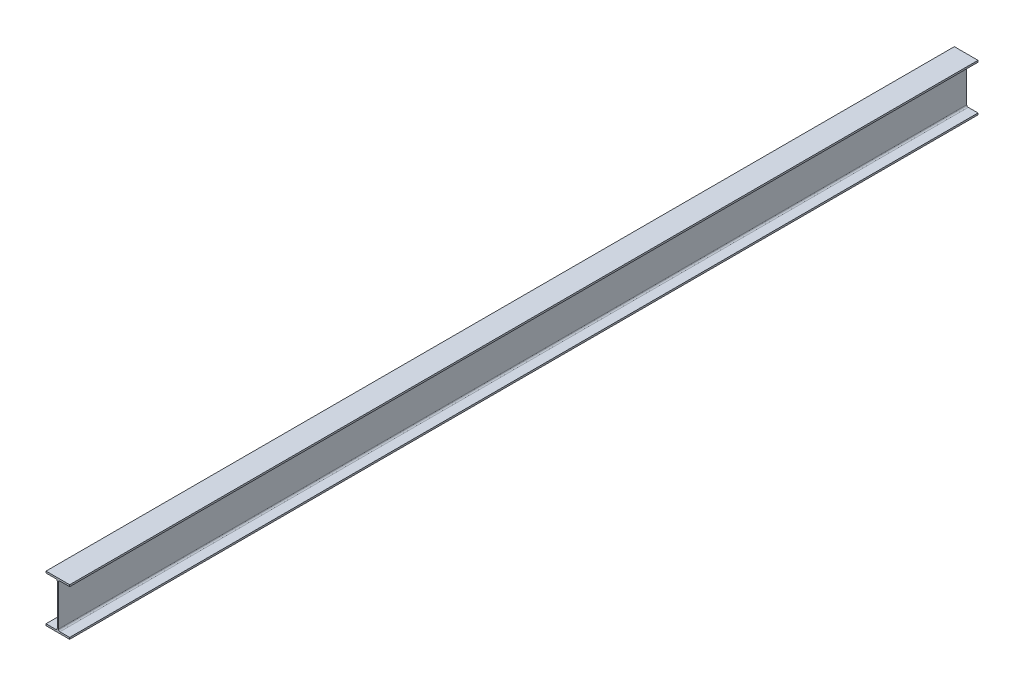
SolidWorks part; units mm, degrees
ref_plane "Front Plane" through (0, 0, 0) normal (0, 0, 1) x (1, 0, 0)
ref_plane "Top Plane" through (0, 0, 0) normal (0, 1, 0) x (1, 0, 0)
ref_plane "Right Plane" through (0, 0, 0) normal (1, 0, 0) x (0, 0, -1)
other "Configuration Table"
sketch "Sketch1" plane through (0, 0, 0) normal (0, 0, 1) x (1, 0, 0)
  line L0 (0, 0) -> (0, 250) construction
  line L1 (62.5, 0) -> (-62.5, 0)
  line L2 (-62.5, 0) -> (-62.5, 9)
  line L3 (-62.5, 9) -> (-11, 9)
  line L4 (3, 17) -> (3, 233)
  line L6 (-62.5, 241) -> (-62.5, 250)
  line L7 (-62.5, 250) -> (62.5, 250)
  line L8 (-3, 17) -> (-3, 233)
  line L9 (62.5, 241) -> (62.5, 250)
  line L10 (11, 241) -> (62.5, 241)
  line L11 (62.5, 9) -> (11, 9)
  line L12 (62.5, 0) -> (62.5, 9)
  line L13 (-11, 241) -> (-62.5, 241)
  arc A0 (11, 9) -> (3, 17) centre (11, 17) cw
  arc A1 (-3, 17) -> (-11, 9) centre (-11, 17) cw
  arc A2 (3, 233) -> (11, 241) centre (11, 233) cw
  arc A3 (-3, 233) -> (-11, 241) centre (-11, 233) ccw
  point P18 (3, 9)
  point P21 (-3, 9)
  point P24 (3, 241)
  point P27 (-3, 241)
  dimension "D6" = 8
  dimension "D1" = 250
  dimension "D2" = 125
  dimension "D3" = 6
  dimension "D4" = 9
  dimension "D5" = 9
extrude "Boss-Extrude1" add sketch "Sketch1" along normal blind 4800
